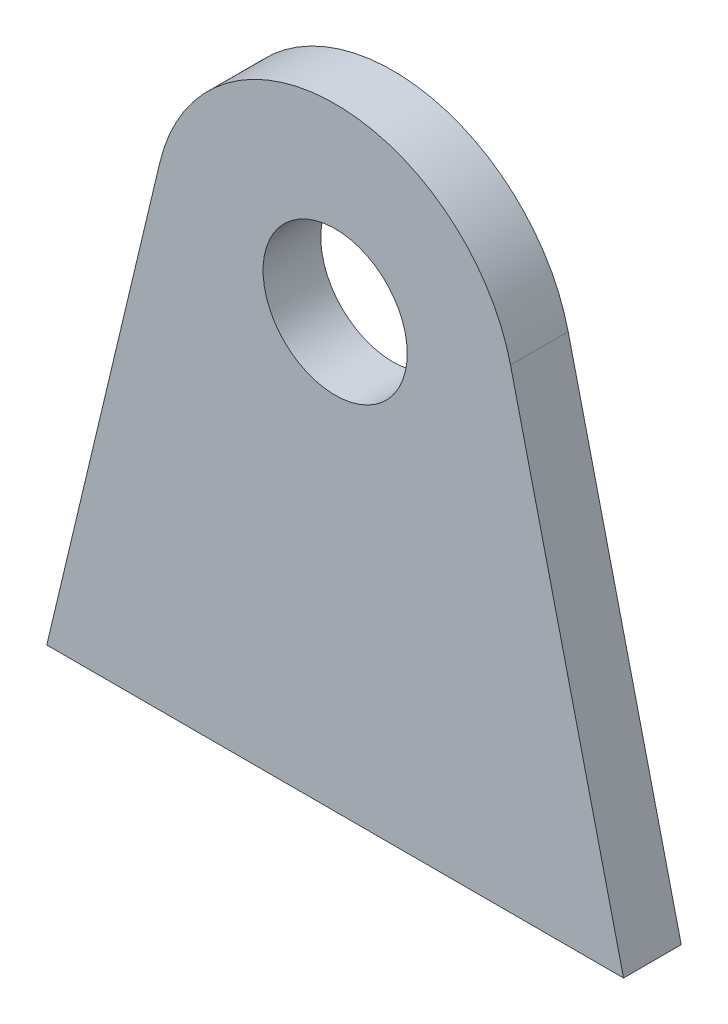
from build123d import *

# Parameters (mm, degrees)
SKETCH_1_R      = 10
EXTRUDE_1_DEPTH = 8


with BuildPart() as part:
    # 草图1 → 凸台-拉伸1 (new body)
    with BuildSketch(Plane.XY):
        with BuildLine():
            Line((0, 0), (80, 0))
            Line((80, 0), (64.318869123, 65.795912749))
            ThreePointArc((64.318869123, 65.795912749), (40, 85), (15.681130877, 65.795912749))
            Line((15.681130877, 65.795912749), (0, 0))
        make_face()
        with Locations((40, 60)):
            Circle(SKETCH_1_R, mode=Mode.SUBTRACT)
    extrude(amount=EXTRUDE_1_DEPTH)


solid = part.part
